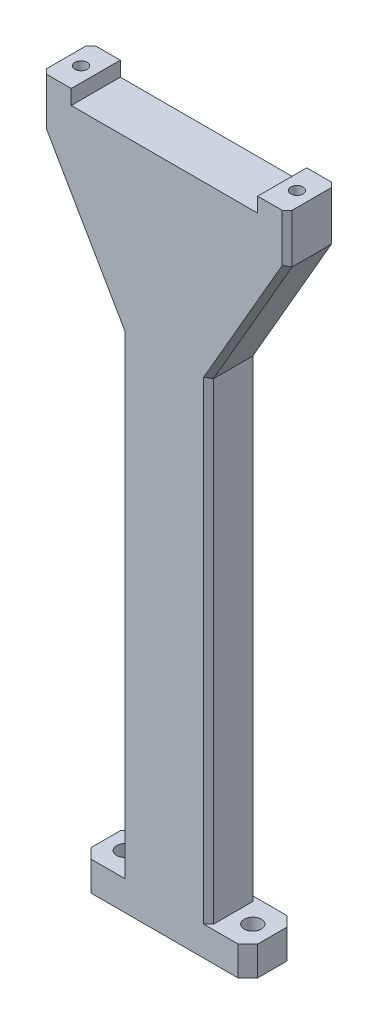
from build123d import *

# Parameters (mm, degrees)
SKETCH1_W                      = 50
SKETCH1_H                      = 140
BOSS_EXTRUDE1_DEPTH            = 5
CUT_EXTRUDE1_DEPTH             = 76
SKETCH3_W                      = 38
SKETCH3_H                      = 3
CUT_EXTRUDE2_DEPTH             = 76
M3_TAPPED_HOLE1_D              = 2.5
M3_TAPPED_HOLE1_DEPTH          = 8.5
M3_TAPPED_HOLE1_TIP            = 0.751075774
F_3_5_3_5_DIAMETER_HOLE1_D     = 3.5
F_3_5_3_5_DIAMETER_HOLE1_DEPTH = 6
CHAMFER1_SIZE                  = 2
CHAMFER2_SIZE                  = 1


with BuildPart() as part:
    # Sketch1 → Boss-Extrude1 (new, symmetric)
    with BuildSketch(Plane.XY):
        Rectangle(SKETCH1_W, SKETCH1_H)
    extrude(amount=BOSS_EXTRUDE1_DEPTH, both=True)

    # Sketch2 → Cut-Extrude1 (cut, through all)
    with BuildSketch(Plane.XY.offset(5)):
        Polygon((-25, 60), (-9, 32.287187079), (-9, -64), (-17, -64), (-17, -70), (-25, -70), align=None)
    cut_extrude1 = extrude(amount=-CUT_EXTRUDE1_DEPTH, mode=Mode.SUBTRACT)

    # Mirror1: Cut-Extrude1 across plane
    add(cut_extrude1.mirror(Plane(origin=(0, 0, 0), x_dir=(0, 0, 1), z_dir=(1, 0, 0))), mode=Mode.SUBTRACT)

    # Sketch3 → Cut-Extrude2 (cut, through all)
    with BuildSketch(Plane.XY.offset(5)):
        with Locations((0, 68.5)):
            Rectangle(SKETCH3_W, SKETCH3_H)
    extrude(amount=-CUT_EXTRUDE2_DEPTH, mode=Mode.SUBTRACT)

    # M3 Tapped Hole1
    with Locations(Plane(origin=(0, 70, 0), x_dir=(1, 0, 0), z_dir=(0, 1, 0))):
        with Locations((-22, 0), (22, 0)):
            Hole(M3_TAPPED_HOLE1_D / 2, depth=M3_TAPPED_HOLE1_DEPTH)
            with Locations((0, 0, -(M3_TAPPED_HOLE1_DEPTH + M3_TAPPED_HOLE1_TIP / 2))):  # 118° drill point
                Cone(0, M3_TAPPED_HOLE1_D / 2, M3_TAPPED_HOLE1_TIP, mode=Mode.SUBTRACT)

    # Ø3.5 (3.5) Diameter Hole1
    with Locations(Plane(origin=(0, -70, 0), x_dir=(-1, 0, 0), z_dir=(0, -1, 0))):
        with Locations((13, 0), (-13, 0)):
            Hole(F_3_5_3_5_DIAMETER_HOLE1_D / 2, depth=F_3_5_3_5_DIAMETER_HOLE1_DEPTH)

    # Chamfer1
    chamfer1_edges = [part.edges().sort_by_distance(p)[0] for p in [
        (-17, -67, -5),
        (-17, -67, 5),
        (17, -67, 5),
        (17, -67, -5),
    ]]
    chamfer(chamfer1_edges, length=CHAMFER1_SIZE)

    # Chamfer2
    chamfer2_edges = [part.edges().sort_by_distance(p)[0] for p in [
        (-25, 65, 5),
        (-17, 46.143593539, -5),
        (-9, -15.856406461, -5),
        (-9, -15.856406461, 5),
        (-17, 46.143593539, 5),
        (25, 65, -5),
        (25, 65, 5),
        (9, -15.856406461, 5),
        (17, 46.143593539, 5),
        (9, -15.856406461, -5),
        (17, 46.143593539, -5),
        (-25, 65, -5),
    ]]
    chamfer(chamfer2_edges, length=CHAMFER2_SIZE)


solid = part.part
